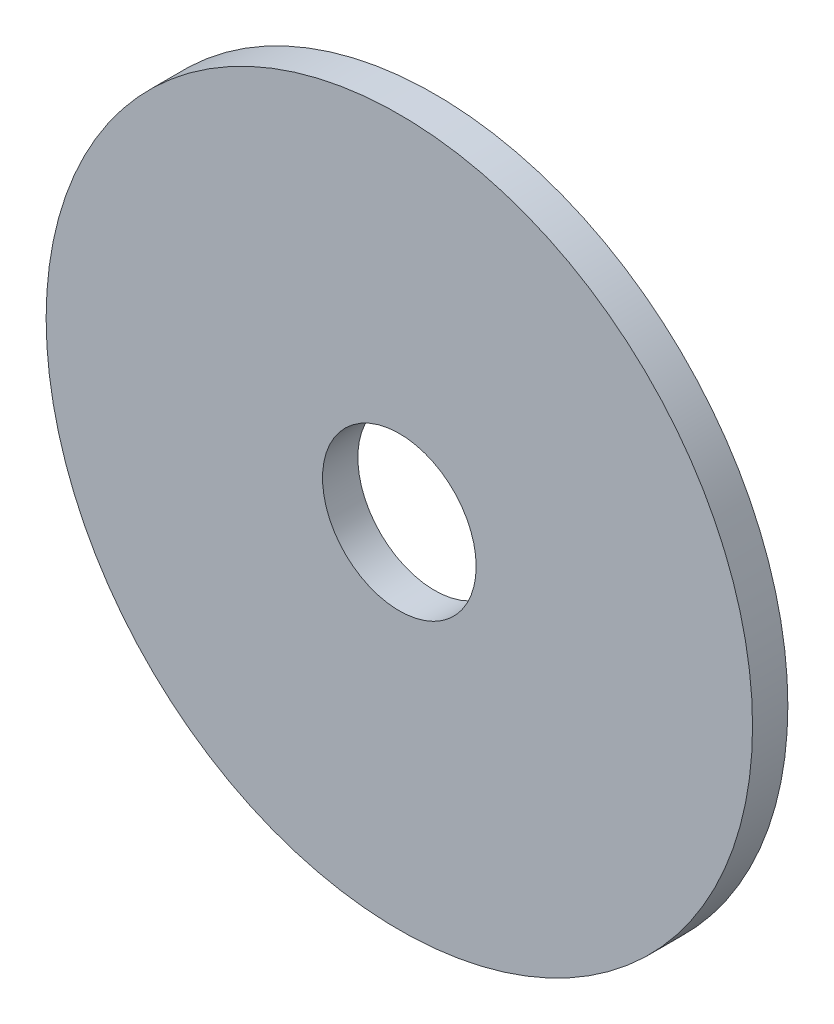
from build123d import *

# Parameters (mm, degrees)
SKETCH_1_R      = 100
SKETCH_1_R_2    = 21.75
EXTRUDE_1_DEPTH = 10


with BuildPart() as part:
    # 草图1 → 凸台-拉伸1 (new body)
    with BuildSketch(Plane.XY):
        Circle(SKETCH_1_R)
        Circle(SKETCH_1_R_2, mode=Mode.SUBTRACT)
    extrude(amount=EXTRUDE_1_DEPTH)


solid = part.part
